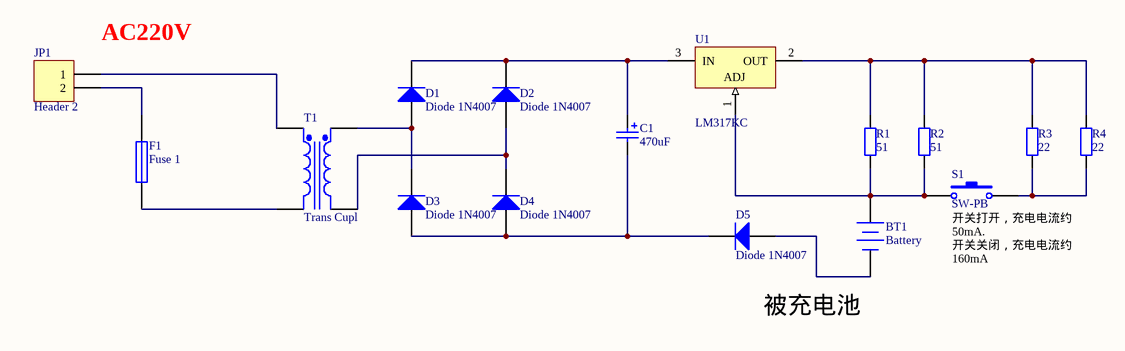
[diagram p0: MISC95143.SCHDOC]
# Altium project MISC95143.PRJPCB
1 sheet, 16 parts. Net scope: global (net labels, ports and power ports of the same name join across sheets).
Board file: MISC95143.PCBDOC

## Sheet MISC95143.SCHDOC
size A4

### Parts
BT1  Battery  [BAT-2]
C1  value 470uF  [RB7.6-15]  (hidden comment: Cap Pol1)
D1  Diode 1N4007  [DIO10.46-5.3x2.8]
D2  Diode 1N4007  [DIO10.46-5.3x2.8]
D3  Diode 1N4007  [DIO10.46-5.3x2.8]
D4  Diode 1N4007  [DIO10.46-5.3x2.8]
D5  Diode 1N4007  [DIO10.46-5.3x2.8]
F1  Fuse 1  [PIN-W2/E2.8]
JP1  Header 2  [HDR1X2]
R1  value 51  [AXIAL-0.4]  (hidden comment: Res2)
R2  value 51  [AXIAL-0.4]  (hidden comment: Res2)
R3  value 22  [AXIAL-0.4]  (hidden comment: Res2)
R4  value 22  [AXIAL-0.4]  (hidden comment: Res2)
S1  SW-PB  [SPST-2]
T1  Trans Cupl  [TRF_4]
U1  LM317KC  [KC03]

### Nets
NetBT1_1: BT1.1(+) R1.1 R2.1 S1.1 U1.1(ADJ)
NetBT1_2: BT1.2(-) D5.1(A)
NetC1_1: C1.1 D1.2(K) D2.2(K) U1.3(IN)
NetC1_2: C1.2 D3.1(A) D4.1(A) D5.2(K)
NetD1_1: D1.1(A) D3.2(K) T1.3(Sec+)
NetD2_1: D2.1(A) D4.2(K) T1.4(Sec-)
NetF1_1: F1.1 T1.2(Pri-)
NetF1_2: F1.2 JP1.2
NetJP1_1: JP1.1 T1.1(Pri+)
NetR1_2: R1.2 R2.2 R3.2 R4.2 U1.2(OUT)
NetR3_1: R3.1 R4.1 S1.2

### Notes on the sheet
- (near JP1) AC220V
- 被充电池
- (near S1) 开关打开，充电电流约50mA.
  开关关闭，充电电流约160mA

### Library data of the parts
BT1 = Battery: Multicell Battery; Published: 24-Mar-1999; Revision: July-2002: Re-released for DXP Platform.; Publisher: Altium Limited
C1 = Cap Pol1: Polarized Capacitor (Radial); Published: 8-Jun-2000; Revision: July-2002: Re-released for DXP Platform.; Publisher: Altium Limited
D1-D5 = Diode 1N4007: 1 Amp General Purpose Rectifier; Revision 1: 11-Jul-2000: SIM Model Added.; Revision 2: 17-Jul-2002: Re-released for DXP Platform.; Package Information: Latest Revision: Aug-1999; Code - JEDEC: DO-204-AL; Published: 8-Jun-2000; Datasheet: Latest Revision: 1998; Package Reference: DO-41; Publisher: Altium Limited
F1 = Fuse 1: Fuse; Published: 8-Jun-2000; Revision: July-2002: Re-released for DXP Platform.; Publisher: Altium Limited
JP1 = Header 2: Header, 2-Pin; Revision: 17-Jul-2002: Re-released for DXP Platform.; Publisher: Altium Limited
R1-R4 = Res2: Resistor; Published: 8-Jun-2000; Revision: July-2002: Re-released for DXP Platform.; Publisher: Altium Limited
S1 = SW-PB: Switch; Published: 24-Mar-1999; Revision: July-2002: Re-released for DXP Platform.; Publisher: Altium Limited
T1 = Trans Cupl: Transformer (Coupled Inductor Model); Published: 8-Jun-2000; Revision: July-2002: Re-released for DXP Platform.; Publisher: Altium Limited
U1 = LM317KC: 3-Terminal Adjustable Regulator; Package Information: Latest Revision: Sep-1995; Note: Pin 2 is electrically connected to tab; Published: 15-Apr-2002; Datasheet: Linear Circuits Data Book 1989 Volume 3 (Feb-1988); Package Reference: KC03; Publisher: Altium Limited